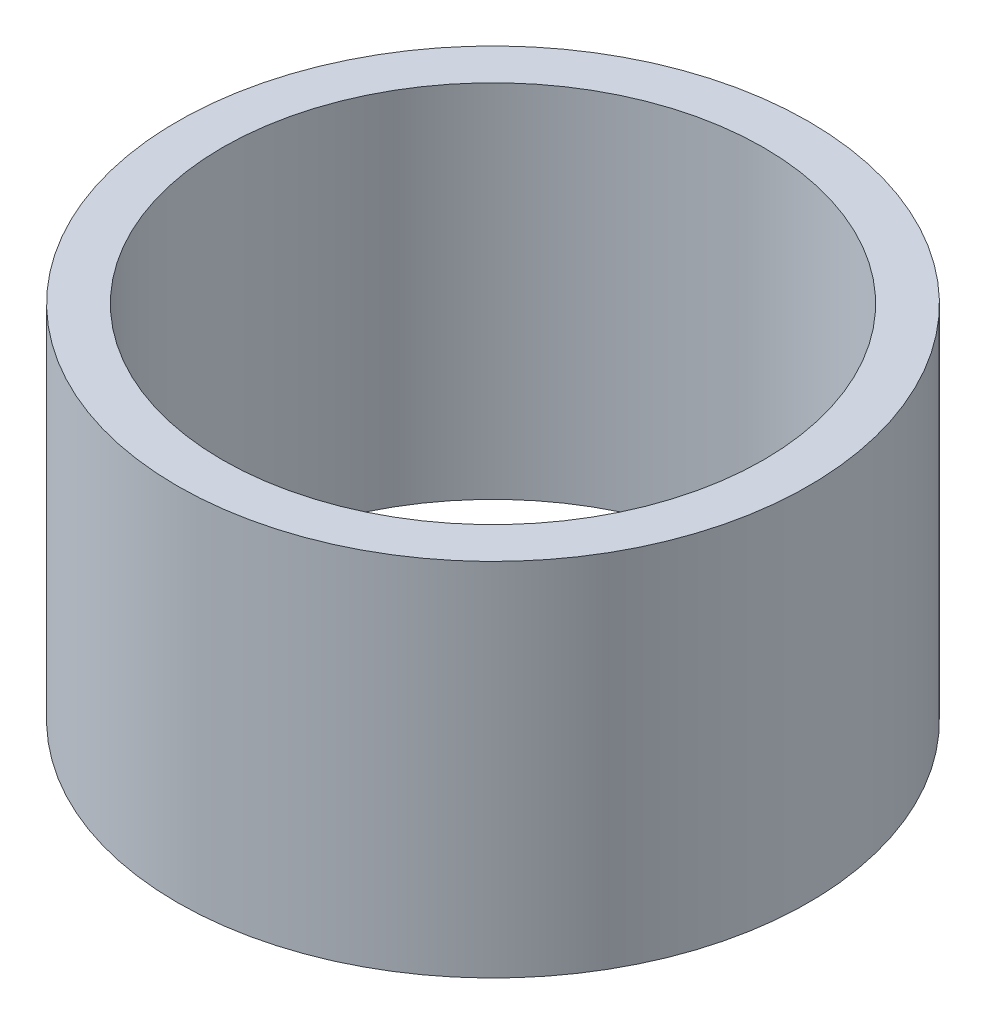
from build123d import *

# Parameters (mm, degrees)
SKETCH1_R           = 7
SKETCH1_R_2         = 6
BOSS_EXTRUDE1_DEPTH = 8


with BuildPart() as part:
    # Sketch1 → Boss-Extrude1 (new body)
    with BuildSketch(Plane(origin=(0, 0, 0), x_dir=(1, 0, 0), z_dir=(0, 1, 0))):
        with Locations(Location((0, 0, 0), (0, 0, 270))):
            Circle(SKETCH1_R)
        with Locations(Location((0, 0, 0), (0, 0, 270))):
            Circle(SKETCH1_R_2, mode=Mode.SUBTRACT)
    extrude(amount=BOSS_EXTRUDE1_DEPTH)


solid = part.part
